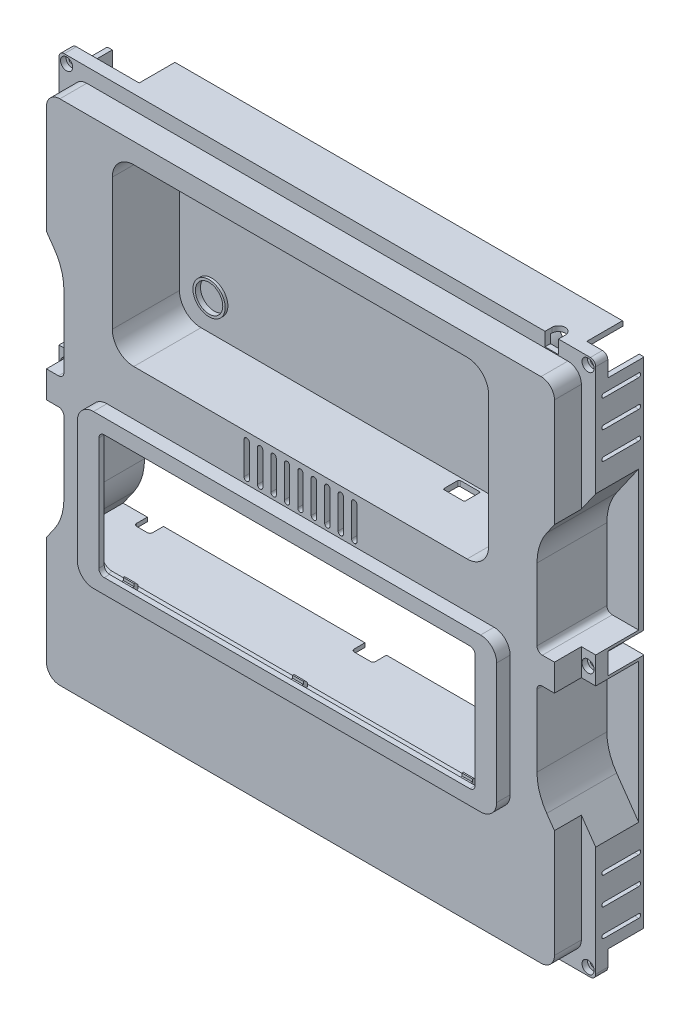
from build123d import *

# Parameters (mm, degrees)
SKETCH1_W                       = 200
SKETCH1_H                       = 200
BOSS_EXTRUDE1_DEPTH             = 18
SKETCH2_W                       = 189
SKETCH2_H                       = 189
BOSS_EXTRUDE2_DEPTH             = 10
CUT_EXTRUDE2_DEPTH              = 30
CUT_EXTRUDE3_DEPTH              = 25
BOSS_EXTRUDE3_DEPTH             = 5
SHELL1_T                        = -2
CUT_EXTRUDE4_DEPTH              = 145.779142144
CUT_EXTRUDE5_DEPTH              = 5.5
CUT_EXTRUDE6_REACH              = 146.167
BOSS_EXTRUDE4_DEPTH             = 26
LPATTERN1_COUNT                 = 5
LPATTERN1_PITCH                 = 5
LPATTERN1_COL_COUNT             = 5
LPATTERN1_COL_PITCH             = 5
SKETCH12_W                      = 12
SKETCH12_H                      = 19.430519509
CUT_EXTRUDE8_DEPTH              = 2
SKETCH13_R                      = 6
SKETCH13_R_2                    = 5.1
BOSS_EXTRUDE5_DEPTH             = 1
SKETCH14_W                      = 16
SKETCH14_H                      = 16
SKETCH14_W_2                    = 18.143709229
SKETCH14_H_2                    = 21.046585881
SKETCH14_W_3                    = 14.115146474
SKETCH14_H_3                    = 23.454738618
CUT_EXTRUDE9_DEPTH              = 13.5
SKETCH15_W                      = 5.5
SKETCH15_H                      = 5.5
SKETCH15_W_2                    = 8
SKETCH15_H_2                    = 10
BOSS_EXTRUDE6_DEPTH             = 2.5
SKETCH16_R                      = 1.1
CUT_EXTRUDE10_DEPTH             = 143.562267098
SKETCH17_W                      = 6
SKETCH17_H                      = 6
BOSS_EXTRUDE7_DEPTH             = 16
CUT_EXTRUDE11_DEPTH             = 145.166570328
CUT_EXTRUDE11_DEPTH_BACK        = 145.166570328
SKETCH18_W                      = 307.102328268
SKETCH18_H                      = 274.194887854
SKETCH18_W_2                    = 199.7
SKETCH18_H_2                    = 199.7
CUT_EXTRUDE12_REACH             = 227.697
SKETCH20_W                      = 12
SKETCH20_H                      = 13.5
CUT_EXTRUDE12_DIRECTION_2_DEPTH = 226.696948362
CUT_EXTRUDE13_REACH             = 227.697
BOSS_EXTRUDE8_DEPTH             = 12
CUT_EXTRUDE14_REACH             = 161.446
CUT_EXTRUDE15_REACH             = 187.944
SKETCH25_W                      = 130
SKETCH25_H                      = 1.5
BOSS_EXTRUDE9_DEPTH             = 2.1
BOSS_EXTRUDE10_DEPTH            = 130
SKETCH27_W                      = 59
SKETCH27_H                      = 52
CUT_EXTRUDE16_DEPTH             = 3.6
BOSS_EXTRUDE13_DEPTH            = 2
SKETCH33_W                      = 7.85
SKETCH33_H                      = 1
BOSS_EXTRUDE19_DEPTH            = 13.5
SKETCH34_R                      = 2.25
CUT_EXTRUDE18_DEPTH             = 2
FILLET1_R                       = 5
FILLET2_R                       = 2
FILLET3_R                       = 2
CHAMFER1_SIZE                   = 0.2
CUT_EXTRUDE19_START             = -0.9
SKETCH35_R                      = 5.1
CUT_EXTRUDE19_DEPTH             = 0.9
SKETCH36_W                      = 13.5
SKETCH36_H                      = 1.85
CUT_EXTRUDE20_DEPTH             = 3
CUT_EXTRUDE21_DEPTH             = 5
SKETCH38_W                      = 4
SKETCH38_H                      = 0.5
BOSS_EXTRUDE20_DEPTH            = 2
SKETCH39_W                      = 0.682359537
SKETCH39_H                      = 8
SKETCH39_W_2                    = 0.830667319
CUT_EXTRUDE22_DEPTH             = 2


with BuildPart() as part:
    # Sketch1 → Boss-Extrude1 (new body)
    with BuildSketch(Plane.XY):
        Rectangle(SKETCH1_W, SKETCH1_H)
    extrude(amount=BOSS_EXTRUDE1_DEPTH)

    # Sketch2 → Boss-Extrude2 (add)
    with BuildSketch(Plane.XY.offset(18)):
        Rectangle(SKETCH2_W, SKETCH2_H)
    extrude(amount=BOSS_EXTRUDE2_DEPTH)

    # Sketch3 → Cut-Extrude2 (cut)
    with BuildSketch(Plane.XY.offset(28)):
        with BuildLine():
            Line((-88, 33.694024222), (-88, 5))
            Line((-88, 5), (-101.930115176, 5))
            Line((-101.930115176, 5), (-101.930115176, -5))
            Line((-101.930115176, -5), (-88, -5))
            Line((-88, -5), (-88, -33.694024222))
            ThreePointArc((-88, -33.694024222), (-88.925660985, -39.708140213), (-91.616959114, -45.165552949))
            Line((-91.616959114, -45.165552949), (-112.611193654, -75.14842716))
            Line((-112.611193654, -75.14842716), (-112.611193654, 75.14842716))
            Line((-112.611193654, 75.14842716), (-91.616959114, 45.165552949))
            ThreePointArc((-91.616959114, 45.165552949), (-88.925660985, 39.708140213), (-88, 33.694024222))
        make_face()
        with BuildLine():
            Line((112.611193654, 75.14842716), (91.616959114, 45.165552949))
            ThreePointArc((91.616959114, 45.165552949), (88.925660985, 39.708140213), (88, 33.694024222))
            Line((88, 33.694024222), (88, 5))
            Line((88, 5), (101.930115176, 5))
            Line((101.930115176, 5), (101.930115176, -5))
            Line((101.930115176, -5), (88, -5))
            Line((88, -5), (88, -33.694024222))
            ThreePointArc((88, -33.694024222), (88.925660985, -39.708140213), (91.616959114, -45.165552949))
            Line((91.616959114, -45.165552949), (112.611193654, -75.14842716))
            Line((112.611193654, -75.14842716), (112.611193654, 75.14842716))
        make_face()
    extrude(amount=-CUT_EXTRUDE2_DEPTH, mode=Mode.SUBTRACT)

    # Sketch4 → Cut-Extrude3 (cut)
    with BuildSketch(Plane.XY.offset(28)):
        with BuildLine():
            Line((-62, 87), (62, 87))
            ThreePointArc((62, 87), (67.656854249, 84.656854249), (70, 79))
            Line((70, 79), (70, 30))
            ThreePointArc((70, 30), (67.656854249, 24.343145751), (62, 22))
            Line((62, 22), (-62, 22))
            ThreePointArc((-62, 22), (-67.656854249, 24.343145751), (-70, 30))
            Line((-70, 30), (-70, 79))
            ThreePointArc((-70, 79), (-67.656854249, 84.656854249), (-62, 87))
        make_face()
    extrude(amount=-CUT_EXTRUDE3_DEPTH, mode=Mode.SUBTRACT)

    # Sketch5 → Boss-Extrude3 (add)
    with BuildSketch(Plane.XY.offset(28)):
        with BuildLine():
            Line((-72, 5), (72, 5))
            ThreePointArc((72, 5), (76.242640687, 3.242640687), (78, -1))
            Line((78, -1), (78, -46))
            ThreePointArc((78, -46), (76.242640687, -50.242640687), (72, -52))
            Line((72, -52), (-72, -52))
            ThreePointArc((-72, -52), (-76.242640687, -50.242640687), (-78, -46))
            Line((-78, -46), (-78, -1))
            ThreePointArc((-78, -1), (-76.242640687, 3.242640687), (-72, 5))
        make_face()
    extrude(amount=BOSS_EXTRUDE3_DEPTH)

    # Shell1
    shell1_openings = [part.faces().sort_by_distance(p)[0] for p in [
        (0, 0, 0),
    ]]
    offset(amount=SHELL1_T, openings=shell1_openings, kind=Kind.INTERSECTION)

    # Sketch6 → Cut-Extrude4 (cut, through all)
    with BuildSketch(Plane(origin=(0, 0, 31), x_dir=(-1, 0, 0), z_dir=(0, 0, -1))):
        with BuildLine():
            Line((-68, -0.5), (68, -0.5))
            ThreePointArc((68, -0.5), (69.414213562, -1.085786438), (70, -2.5))
            Line((70, -2.5), (70, -44.5))
            ThreePointArc((70, -44.5), (69.414213562, -45.914213562), (68, -46.5))
            Line((68, -46.5), (-68, -46.5))
            ThreePointArc((-68, -46.5), (-69.414213562, -45.914213562), (-70, -44.5))
            Line((-70, -44.5), (-70, -2.5))
            ThreePointArc((-70, -2.5), (-69.414213562, -1.085786438), (-68, -0.5))
        make_face()
    extrude(amount=-CUT_EXTRUDE4_DEPTH, mode=Mode.SUBTRACT)

    # Sketch7 → Cut-Extrude5 (cut)
    with BuildSketch(Plane(origin=(0, 100, 0), x_dir=(1, 0, 0), z_dir=(0, 1, 0))):
        with BuildLine():
            Line((-88, -9), (-79, -9))
            ThreePointArc((-79, -9), (-77.939339828, -9.439339828), (-77.5, -10.5))
            Line((-77.5, -10.5), (-77.5, -13.5))
            Line((-77.5, -13.5), (-81, -13.5))
            Line((-81, -13.5), (-89.5, -13.5))
            Line((-89.5, -13.5), (-89.5, -10.5))
            ThreePointArc((-89.5, -10.5), (-89.060660172, -9.439339828), (-88, -9))
        make_face()
    extrude(amount=-CUT_EXTRUDE5_DEPTH, mode=Mode.SUBTRACT)

    # Sketch9 → Cut-Extrude6 (cut, up to next)
    with BuildSketch(Plane.XY.offset(28), mode=Mode.PRIVATE) as cut_extrude6_sk1:
        with BuildLine():
            Line((1, 19), (1, 7))
            ThreePointArc((1, 7), (0, 6), (-1, 7))
            Line((-1, 7), (-1, 19))
            ThreePointArc((-1, 19), (0, 20), (1, 19))
        make_face()
    cut_extrude6_tool1 = extrude(cut_extrude6_sk1.sketch, amount=-CUT_EXTRUDE6_REACH, mode=Mode.PRIVATE) & part.part
    cut_extrude6 = cut_extrude6_tool1.solids().sort_by_distance((0, 13, 28))[0]
    add(cut_extrude6, mode=Mode.SUBTRACT)

    # Sketch10 → Boss-Extrude4 (add)
    with BuildSketch(Plane(origin=(0, 0, 26), x_dir=(-1, 0, 0), z_dir=(0, 0, -1))):
        Polygon((-94.530667319, -52), (-95.330667319, -52.8), (-95.330667319, -53.5), (95.182359537, -53.5), (95.182359537, -52.8), (94.382359537, -52), align=None)
    extrude(amount=BOSS_EXTRUDE4_DEPTH)

    # LPattern1: Cut-Extrude6 ×5
    with Locations(*[(i * LPATTERN1_PITCH, 0, 0) for i in range(1, LPATTERN1_COUNT)]):
        add(cut_extrude6, mode=Mode.SUBTRACT)

    # LPattern1 col: Cut-Extrude6 ×5
    with Locations(*[(-i * LPATTERN1_COL_PITCH, 0, 0) for i in range(1, LPATTERN1_COL_COUNT)]):
        add(cut_extrude6, mode=Mode.SUBTRACT)

    # Sketch12 → Cut-Extrude8 (cut)
    with BuildSketch(Plane(origin=(0, 100, 0), x_dir=(1, 0, 0), z_dir=(0, 1, 0))):
        with Locations((-83.5, -2.284740245)):
            Rectangle(SKETCH12_W, SKETCH12_H)
    extrude(amount=-CUT_EXTRUDE8_DEPTH, mode=Mode.SUBTRACT)

    # Sketch13 → Boss-Extrude5 (add)
    # profile 1 of 4: a face of its own
    with BuildSketch(Plane.XY.offset(3)):
        with Locations((-58, 75)):
            Circle(SKETCH13_R)
        with Locations((-58, 75)):
            Circle(SKETCH13_R_2, mode=Mode.SUBTRACT)
    # profile 2 of 4: a face of its own
    with BuildSketch(Plane.XY.offset(3)):
        with Locations((-58, 34)):
            Circle(SKETCH13_R)
        with Locations((-58, 34)):
            Circle(SKETCH13_R_2, mode=Mode.SUBTRACT)
    # profile 3 of 4: a face of its own
    with BuildSketch(Plane.XY.offset(3)):
        with Locations((58, 34)):
            Circle(SKETCH13_R)
        with Locations((58, 34)):
            Circle(SKETCH13_R_2, mode=Mode.SUBTRACT)
    # profile 4 of 4: a face of its own
    with BuildSketch(Plane.XY.offset(3)):
        with Locations((58, 75)):
            Circle(SKETCH13_R)
        with Locations((58, 75)):
            Circle(SKETCH13_R_2, mode=Mode.SUBTRACT)
    extrude(amount=BOSS_EXTRUDE5_DEPTH)

    # Sketch14 → Cut-Extrude9 (cut)
    with BuildSketch(Plane(origin=(0, 0, 0), x_dir=(-1, 0, 0), z_dir=(0, 0, -1))):
        with Locations((100, 100)):
            Rectangle(SKETCH14_W, SKETCH14_H)
        with Locations((-100, 100)):
            Rectangle(SKETCH14_W, SKETCH14_H)
        with Locations((100, -100)):
            Rectangle(SKETCH14_W, SKETCH14_H)
        with Locations((-100, -100)):
            Rectangle(SKETCH14_W, SKETCH14_H)
        with Locations((-101.071854615, 0.410400912)):
            Rectangle(SKETCH14_W_2, SKETCH14_H_2)
        with Locations((99.057573237, 1.61447728)):
            Rectangle(SKETCH14_W_3, SKETCH14_H_3)
    extrude(amount=-CUT_EXTRUDE9_DEPTH, mode=Mode.SUBTRACT)

    # Sketch15 → Boss-Extrude6 (add)
    with BuildSketch(Plane(origin=(0, 0, 16), x_dir=(-1, 0, 0), z_dir=(0, 0, -1))):
        with Locations((-95.25, 95.25)):
            Rectangle(SKETCH15_W, SKETCH15_H)
        with Locations((95.25, 95.25)):
            Rectangle(SKETCH15_W, SKETCH15_H)
        with Locations((95.25, -95.25)):
            Rectangle(SKETCH15_W, SKETCH15_H)
        with Locations((-95.25, -95.25)):
            Rectangle(SKETCH15_W, SKETCH15_H)
        with Locations((-96, 0)):
            Rectangle(SKETCH15_W_2, SKETCH15_H_2)
        with Locations((96, 0)):
            Rectangle(SKETCH15_W_2, SKETCH15_H_2)
    extrude(amount=BOSS_EXTRUDE6_DEPTH)

    # Sketch16 → Cut-Extrude10 (cut, through all)
    with BuildSketch(Plane.XY.offset(18)):
        with Locations((-97, 97)):
            Circle(SKETCH16_R)
        with Locations((97, 97)):
            Circle(SKETCH16_R)
        with Locations((97, -97)):
            Circle(SKETCH16_R)
        with Locations((-97, -97)):
            Circle(SKETCH16_R)
        with Locations((-97, 0)):
            Circle(SKETCH16_R)
        with Locations((97, 0)):
            Circle(SKETCH16_R)
    extrude(amount=-CUT_EXTRUDE10_DEPTH, mode=Mode.SUBTRACT)

    # Sketch17 → Boss-Extrude7 (add)
    with BuildSketch(Plane(origin=(0, 0, 0), x_dir=(-1, 0, 0), z_dir=(0, 0, -1))):
        with Locations((89, 0)):
            Rectangle(SKETCH17_W, SKETCH17_H)
        with Locations((-89, 0)):
            Rectangle(SKETCH17_W, SKETCH17_H)
    extrude(amount=-BOSS_EXTRUDE7_DEPTH)

    # Sketch18 → Cut-Extrude11 (cut, two sides: drawn at the far end of the back side and taken through both)
    with BuildSketch(Plane.XY.offset(28).offset(-CUT_EXTRUDE11_DEPTH_BACK)):
        Rectangle(SKETCH18_W, SKETCH18_H)
        Rectangle(SKETCH18_W_2, SKETCH18_H_2, mode=Mode.SUBTRACT)
    extrude(amount=CUT_EXTRUDE11_DEPTH + CUT_EXTRUDE11_DEPTH_BACK, mode=Mode.SUBTRACT)

    # Sketch20 → Cut-Extrude12 (cut, up to next)
    with BuildSketch(Plane(origin=(0, 99.85, 0), x_dir=(1, 0, 0), z_dir=(0, 1, 0)), mode=Mode.PRIVATE) as cut_extrude12_sk1:
        with Locations((-92, -6.75)):
            Rectangle(SKETCH20_W, SKETCH20_H)
    cut_extrude12_tool1 = extrude(cut_extrude12_sk1.sketch, amount=-CUT_EXTRUDE12_REACH, mode=Mode.PRIVATE) & part.part
    add(cut_extrude12_tool1.solids().sort_by_distance((-92, 99.85, 6.75))[0], mode=Mode.SUBTRACT)

    # Sketch20 → Cut-Extrude12 direction 2 (cut)
    with BuildSketch(Plane(origin=(0, 99.85, 0), x_dir=(1, 0, 0), z_dir=(0, 1, 0))):
        with Locations((-92, -6.75)):
            Rectangle(SKETCH20_W, SKETCH20_H)
    extrude(amount=CUT_EXTRUDE12_DIRECTION_2_DEPTH, mode=Mode.SUBTRACT)

    # Sketch21 → Cut-Extrude13 (cut, up to next)
    with BuildSketch(Plane(origin=(99.85, 0, 0), x_dir=(0, 0, -1), z_dir=(1, 0, 0)), mode=Mode.PRIVATE) as cut_extrude13_sk1:
        with BuildLine():
            Line((-15, 87.85), (-2, 87.85))
            ThreePointArc((-2, 87.85), (-1.25, 87.1), (-2, 86.35))
            Line((-2, 86.35), (-15, 86.35))
            ThreePointArc((-15, 86.35), (-15.75, 87.1), (-15, 87.85))
        make_face()
    cut_extrude13_tool1 = extrude(cut_extrude13_sk1.sketch, amount=-CUT_EXTRUDE13_REACH, mode=Mode.PRIVATE) & part.part
    # Sketch21 → Cut-Extrude13 (cut, up to next)
    with BuildSketch(Plane(origin=(99.85, 0, 0), x_dir=(0, 0, -1), z_dir=(1, 0, 0)), mode=Mode.PRIVATE) as cut_extrude13_sk2:
        with BuildLine():
            Line((-15, 77.63), (-2, 77.63))
            ThreePointArc((-2, 77.63), (-1.25, 76.88), (-2, 76.13))
            Line((-2, 76.13), (-15, 76.13))
            ThreePointArc((-15, 76.13), (-15.75, 76.88), (-15, 77.63))
        make_face()
    cut_extrude13_tool2 = extrude(cut_extrude13_sk2.sketch, amount=-CUT_EXTRUDE13_REACH, mode=Mode.PRIVATE) & part.part
    # Sketch21 → Cut-Extrude13 (cut, up to next)
    with BuildSketch(Plane(origin=(99.85, 0, 0), x_dir=(0, 0, -1), z_dir=(1, 0, 0)), mode=Mode.PRIVATE) as cut_extrude13_sk3:
        with BuildLine():
            Line((-15, -87.85), (-2, -87.85))
            ThreePointArc((-2, -87.85), (-1.25, -87.1), (-2, -86.35))
            Line((-2, -86.35), (-15, -86.35))
            ThreePointArc((-15, -86.35), (-15.75, -87.1), (-15, -87.85))
        make_face()
    cut_extrude13_tool3 = extrude(cut_extrude13_sk3.sketch, amount=-CUT_EXTRUDE13_REACH, mode=Mode.PRIVATE) & part.part
    # Sketch21 → Cut-Extrude13 (cut, up to next)
    with BuildSketch(Plane(origin=(99.85, 0, 0), x_dir=(0, 0, -1), z_dir=(1, 0, 0)), mode=Mode.PRIVATE) as cut_extrude13_sk4:
        with BuildLine():
            Line((-15, -77.63), (-2, -77.63))
            ThreePointArc((-2, -77.63), (-1.25, -76.88), (-2, -76.13))
            Line((-2, -76.13), (-15, -76.13))
            ThreePointArc((-15, -76.13), (-15.75, -76.88), (-15, -77.63))
        make_face()
    cut_extrude13_tool4 = extrude(cut_extrude13_sk4.sketch, amount=-CUT_EXTRUDE13_REACH, mode=Mode.PRIVATE) & part.part
    # Sketch21 → Cut-Extrude13 (cut, up to next)
    with BuildSketch(Plane(origin=(99.85, 0, 0), x_dir=(0, 0, -1), z_dir=(1, 0, 0)), mode=Mode.PRIVATE) as cut_extrude13_sk5:
        with BuildLine():
            Line((-15, 67.41), (-2, 67.41))
            ThreePointArc((-2, 67.41), (-1.25, 66.66), (-2, 65.91))
            Line((-2, 65.91), (-15, 65.91))
            ThreePointArc((-15, 65.91), (-15.75, 66.66), (-15, 67.41))
        make_face()
    cut_extrude13_tool5 = extrude(cut_extrude13_sk5.sketch, amount=-CUT_EXTRUDE13_REACH, mode=Mode.PRIVATE) & part.part
    # Sketch21 → Cut-Extrude13 (cut, up to next)
    with BuildSketch(Plane(origin=(99.85, 0, 0), x_dir=(0, 0, -1), z_dir=(1, 0, 0)), mode=Mode.PRIVATE) as cut_extrude13_sk6:
        with BuildLine():
            Line((-15, -67.41), (-2, -67.41))
            ThreePointArc((-2, -67.41), (-1.25, -66.66), (-2, -65.91))
            Line((-2, -65.91), (-15, -65.91))
            ThreePointArc((-15, -65.91), (-15.75, -66.66), (-15, -67.41))
        make_face()
    cut_extrude13_tool6 = extrude(cut_extrude13_sk6.sketch, amount=-CUT_EXTRUDE13_REACH, mode=Mode.PRIVATE) & part.part
    cut_extrude13_1 = cut_extrude13_tool1.solids().sort_by_distance((99.85, 87.1, 8.5))[0]
    add(cut_extrude13_1, mode=Mode.SUBTRACT)
    cut_extrude13_2 = cut_extrude13_tool2.solids().sort_by_distance((99.85, 76.88, 8.5))[0]
    add(cut_extrude13_2, mode=Mode.SUBTRACT)
    cut_extrude13_3 = cut_extrude13_tool3.solids().sort_by_distance((99.85, -87.1, 8.5))[0]
    add(cut_extrude13_3, mode=Mode.SUBTRACT)
    cut_extrude13_4 = cut_extrude13_tool4.solids().sort_by_distance((99.85, -76.88, 8.5))[0]
    add(cut_extrude13_4, mode=Mode.SUBTRACT)
    cut_extrude13_5 = cut_extrude13_tool5.solids().sort_by_distance((99.85, 66.66, 8.5))[0]
    add(cut_extrude13_5, mode=Mode.SUBTRACT)
    cut_extrude13_6 = cut_extrude13_tool6.solids().sort_by_distance((99.85, -66.66, 8.5))[0]
    add(cut_extrude13_6, mode=Mode.SUBTRACT)
    cut_extrude13 = cut_extrude13_1 + cut_extrude13_2 + cut_extrude13_3 + cut_extrude13_4 + cut_extrude13_5 + cut_extrude13_6  # Cut-Extrude13 as one shape, for the pattern or mirror that repeats it

    # Mirror1: Cut-Extrude13 across plane
    add(cut_extrude13.mirror(Plane(origin=(0, 0, 0), x_dir=(0, 0, 1), z_dir=(1, 0, 0))), mode=Mode.SUBTRACT)

    # Sketch22 → Boss-Extrude8 (add)
    with BuildSketch(Plane(origin=(0, 0, 26), x_dir=(-1, 0, 0), z_dir=(0, 0, -1))):
        with BuildLine():
            Line((-26, 20), (-26, 8))
            ThreePointArc((-26, 8), (-25.414213562, 6.585786438), (-24, 6))
            Line((-24, 6), (24, 6))
            ThreePointArc((24, 6), (25.414213562, 6.585786438), (26, 8))
            Line((26, 8), (26, 20))
            Line((26, 20), (27, 20))
            Line((27, 20), (27, 8))
            ThreePointArc((27, 8), (26.121320344, 5.878679656), (24, 5))
            Line((24, 5), (-24, 5))
            ThreePointArc((-24, 5), (-26.121320344, 5.878679656), (-27, 8))
            Line((-27, 8), (-27, 20))
            Line((-27, 20), (-26, 20))
        make_face()
    extrude(amount=BOSS_EXTRUDE8_DEPTH)

    # Sketch23 → Cut-Extrude14 (cut, up to next)
    with BuildSketch(Plane(origin=(0, 20, 0), x_dir=(-1, 0, 0), z_dir=(0, -1, 0)), mode=Mode.PRIVATE) as cut_extrude14_sk1:
        with BuildLine():
            Line((-42.5, -4), (-35.5, -4))
            ThreePointArc((-35.5, -4), (-35.146446609, -4.146446609), (-35, -4.5))
            Line((-35, -4.5), (-35, -9.5))
            ThreePointArc((-35, -9.5), (-35.146446609, -9.853553391), (-35.5, -10))
            Line((-35.5, -10), (-42.5, -10))
            ThreePointArc((-42.5, -10), (-42.853553391, -9.853553391), (-43, -9.5))
            Line((-43, -9.5), (-43, -4.5))
            ThreePointArc((-43, -4.5), (-42.853553391, -4.146446609), (-42.5, -4))
        make_face()
    cut_extrude14_tool1 = extrude(cut_extrude14_sk1.sketch, amount=-CUT_EXTRUDE14_REACH, mode=Mode.PRIVATE) & part.part
    add(cut_extrude14_tool1.solids().sort_by_distance((39, 20, 7))[0], mode=Mode.SUBTRACT)

    # Sketch24 → Cut-Extrude15 (cut, up to next)
    with BuildSketch(Plane(origin=(0, -53.5, 0), x_dir=(-1, 0, 0), z_dir=(0, -1, 0)), mode=Mode.PRIVATE) as cut_extrude15_sk1:
        with BuildLine():
            Line((4, 5), (-4, 5))
            Line((-4, 5), (-4, -4))
            ThreePointArc((-4, -4), (-3.707106781, -4.707106781), (-3, -5))
            Line((-3, -5), (3, -5))
            ThreePointArc((3, -5), (3.707106781, -4.707106781), (4, -4))
            Line((4, -4), (4, 5))
        make_face()
    cut_extrude15_tool1 = extrude(cut_extrude15_sk1.sketch, amount=-CUT_EXTRUDE15_REACH, mode=Mode.PRIVATE) & part.part
    # Sketch24 → Cut-Extrude15 (cut, up to next)
    with BuildSketch(Plane(origin=(0, -53.5, 0), x_dir=(-1, 0, 0), z_dir=(0, -1, 0)), mode=Mode.PRIVATE) as cut_extrude15_sk2:
        with BuildLine():
            Line((-84.959446153, 3.048608869), (-78.959446153, 3.048608869))
            Line((-78.959446153, 3.048608869), (-78.959446153, -4))
            ThreePointArc((-78.959446153, -4), (-79.252339372, -4.707106781), (-79.959446153, -5))
            Line((-79.959446153, -5), (-83.959446153, -5))
            ThreePointArc((-83.959446153, -5), (-84.666552934, -4.707106781), (-84.959446153, -4))
            Line((-84.959446153, -4), (-84.959446153, 3.048608869))
        make_face()
    cut_extrude15_tool2 = extrude(cut_extrude15_sk2.sketch, amount=-CUT_EXTRUDE15_REACH, mode=Mode.PRIVATE) & part.part
    # Sketch24 → Cut-Extrude15 (cut, up to next)
    with BuildSketch(Plane(origin=(0, -53.5, 0), x_dir=(-1, 0, 0), z_dir=(0, -1, 0)), mode=Mode.PRIVATE) as cut_extrude15_sk3:
        with BuildLine():
            Line((78.959446153, 3.048608869), (78.959446153, -4))
            ThreePointArc((78.959446153, -4), (79.252339372, -4.707106781), (79.959446153, -5))
            Line((79.959446153, -5), (83.959446153, -5))
            ThreePointArc((83.959446153, -5), (84.666552934, -4.707106781), (84.959446153, -4))
            Line((84.959446153, -4), (84.959446153, 3.048608869))
            Line((84.959446153, 3.048608869), (78.959446153, 3.048608869))
        make_face()
    cut_extrude15_tool3 = extrude(cut_extrude15_sk3.sketch, amount=-CUT_EXTRUDE15_REACH, mode=Mode.PRIVATE) & part.part
    add(cut_extrude15_tool1.solids().sort_by_distance((0, -53.5, -0.025765))[0], mode=Mode.SUBTRACT)
    add(cut_extrude15_tool2.solids().sort_by_distance((81.959446, -53.5, 0.941611))[0], mode=Mode.SUBTRACT)
    add(cut_extrude15_tool3.solids().sort_by_distance((-81.959446, -53.5, 0.941611))[0], mode=Mode.SUBTRACT)

    # Sketch25 → Boss-Extrude9 (add)
    with BuildSketch(Plane(origin=(0, 0, 31), x_dir=(-1, 0, 0), z_dir=(0, 0, -1))):
        with Locations((0, 1.75)):
            Rectangle(SKETCH25_W, SKETCH25_H)
        with Locations((0, -48.75)):
            Rectangle(SKETCH25_W, SKETCH25_H)
    extrude(amount=BOSS_EXTRUDE9_DEPTH)

    # Sketch26 → Boss-Extrude10 (add)
    with BuildSketch(Plane.ZY.offset(65)):
        Polygon((28.9, 1), (28.9, 0), (28.4, 0), (27.4, 1.10248717), (27.4, 2.5), (28.9, 2.5), align=None)
        Polygon((28.9, -49.5), (28.9, -48), (28.9, -47), (28.4, -47), (27.4, -48.10248717), (27.4, -49.5), align=None)
    extrude(amount=-BOSS_EXTRUDE10_DEPTH)

    # Sketch27 → Cut-Extrude16 (cut)
    with BuildSketch(Plane(origin=(0, 0, 27.4), x_dir=(-1, 0, 0), z_dir=(0, 0, -1))):
        with Locations((-31.5, -23.5)):
            Rectangle(SKETCH27_W, SKETCH27_H)
        with Locations((31.5, -23.5)):
            Rectangle(SKETCH27_W, SKETCH27_H)
    extrude(amount=-CUT_EXTRUDE16_DEPTH, mode=Mode.SUBTRACT)

    # Sketch31 → Boss-Extrude13 (add)
    with BuildSketch(Plane(origin=(0, 0, 0), x_dir=(-1, 0, 0), z_dir=(0, 0, -1))):
        Polygon((99.85, 56.92355388), (99.85, 5), (92, 5), (92, -5), (99.85, -5), (99.85, -56.92355388), (87.955798071, -40.983871708), (86.965756204, -34.11545626), (86.965756204, 34.47937736), (88.839200246, 42.456119225), align=None)
        Polygon((-99.85, -5), (-99.85, -56.92355388), (-87.955798071, -40.983871708), (-86.965756204, -34.11545626), (-86.965756204, 34.47937736), (-88.839200246, 42.456119225), (-99.85, 56.92355388), (-99.85, 5), (-92, 5), (-92, -5), align=None)
    extrude(amount=-BOSS_EXTRUDE13_DEPTH)

    # Sketch33 → Boss-Extrude19 (add)
    with BuildSketch(Plane(origin=(0, 0, 13.5), x_dir=(-1, 0, 0), z_dir=(0, 0, -1))):
        with Locations((-95.925, 4.5)):
            Rectangle(SKETCH33_W, SKETCH33_H)
        with Locations((-95.925, -4.5)):
            Rectangle(SKETCH33_W, SKETCH33_H)
        with Locations((95.925, -4.5)):
            Rectangle(SKETCH33_W, SKETCH33_H)
        with Locations((95.925, 4.5)):
            Rectangle(SKETCH33_W, SKETCH33_H)
    extrude(amount=BOSS_EXTRUDE19_DEPTH)

    # Sketch34 → Cut-Extrude18 (cut)
    with BuildSketch(Plane.XY.offset(18)):
        with Locations((97, 97)):
            Circle(SKETCH34_R)
        with Locations((97, 0)):
            Circle(SKETCH34_R)
        with Locations((97, -97)):
            Circle(SKETCH34_R)
        with Locations((-97, -97)):
            Circle(SKETCH34_R)
        with Locations((-97, 0)):
            Circle(SKETCH34_R)
        with Locations((-97, 97)):
            Circle(SKETCH34_R)
    extrude(amount=-CUT_EXTRUDE18_DEPTH, mode=Mode.SUBTRACT)

    # Fillet1
    fillet1_edges = [part.edges().sort_by_distance(p)[0] for p in [
        (94.5, -94.5, 23),
        (94.5, 94.5, 23),
        (-94.5, 94.5, 23),
        (-94.5, -94.5, 23),
    ]]
    fillet(fillet1_edges, radius=FILLET1_R)

    # Fillet2
    fillet2_edges = [part.edges().sort_by_distance(p)[0] for p in [
        (-99.85, -99.85, 15.75),
        (-99.85, 99.85, 15.75),
        (99.85, 99.85, 15.75),
        (99.85, -99.85, 15.75),
    ]]
    fillet(fillet2_edges, radius=FILLET2_R)

    # Fillet3
    fillet3_edges = [part.edges().sort_by_distance(p)[0] for p in [
        (-88, 5, 15),
        (-88, -5, 15),
        (88, -5, 15),
        (88, 5, 15),
    ]]
    fillet(fillet3_edges, radius=FILLET3_R)

    # Chamfer1
    chamfer1_edges = [part.edges().sort_by_distance(p)[0] for p in [
        (-99.85, -48, 0),
        (99.85, -48, 0),
        (0, -99.85, 0),
        (-99.85, 48, 0),
        (99.85, 48, 0),
        (7.25, 99.85, 0),
    ]]
    chamfer(chamfer1_edges, length=CHAMFER1_SIZE)

    # Sketch35 → Cut-Extrude19 (cut)
    with BuildSketch(Plane.XY.offset(3).offset(CUT_EXTRUDE19_START)):
        with Locations((-58, 34)):
            Circle(SKETCH35_R)
        with Locations((-58, 75)):
            Circle(SKETCH35_R)
        with Locations((58, 75)):
            Circle(SKETCH35_R)
        with Locations((58, 34)):
            Circle(SKETCH35_R)
    extrude(amount=CUT_EXTRUDE19_DEPTH, mode=Mode.SUBTRACT)

    # Sketch36 → Cut-Extrude20 (cut)
    with BuildSketch(Plane.ZY.offset(77.5)):
        with Locations((6.75, 98.925)):
            Rectangle(SKETCH36_W, SKETCH36_H)
    extrude(amount=-CUT_EXTRUDE20_DEPTH, mode=Mode.SUBTRACT)

    # Sketch37 → Cut-Extrude21 (cut)
    with BuildSketch(Plane(origin=(0, 99.85, 0), x_dir=(1, 0, 0), z_dir=(0, 1, 0))):
        with BuildLine():
            Line((86, -15.5), (86, -20.387398891))
            ThreePointArc((86, -20.387398891), (83.5, -22.887398891), (81, -20.387398891))
            Line((81, -20.387398891), (81, -15.5))
            ThreePointArc((81, -15.5), (83.5, -13), (86, -15.5))
        make_face()
    extrude(amount=-CUT_EXTRUDE21_DEPTH, mode=Mode.SUBTRACT)

    # Sketch38 → Boss-Extrude20 (add)
    with BuildSketch(Plane(origin=(0, 0, 31), x_dir=(-1, 0, 0), z_dir=(0, 0, -1))):
        with Locations((-63, 2.75)):
            Rectangle(SKETCH38_W, SKETCH38_H)
        with Locations((-63, -49.75)):
            Rectangle(SKETCH38_W, SKETCH38_H)
        with Locations((0, 2.75)):
            Rectangle(SKETCH38_W, SKETCH38_H)
        with Locations((63, 2.75)):
            Rectangle(SKETCH38_W, SKETCH38_H)
        with Locations((0, -49.75)):
            Rectangle(SKETCH38_W, SKETCH38_H)
        with Locations((63, -49.75)):
            Rectangle(SKETCH38_W, SKETCH38_H)
    extrude(amount=BOSS_EXTRUDE20_DEPTH)

    # Sketch39 → Cut-Extrude22 (cut)
    with BuildSketch(Plane(origin=(0, -53.5, 0), x_dir=(-1, 0, 0), z_dir=(0, -1, 0))):
        with Locations((94.841179769, -22)):
            Rectangle(SKETCH39_W, SKETCH39_H)
        with Locations((-94.915333659, -22)):
            Rectangle(SKETCH39_W_2, SKETCH39_H)
    extrude(amount=-CUT_EXTRUDE22_DEPTH, mode=Mode.SUBTRACT)


solid = part.part
